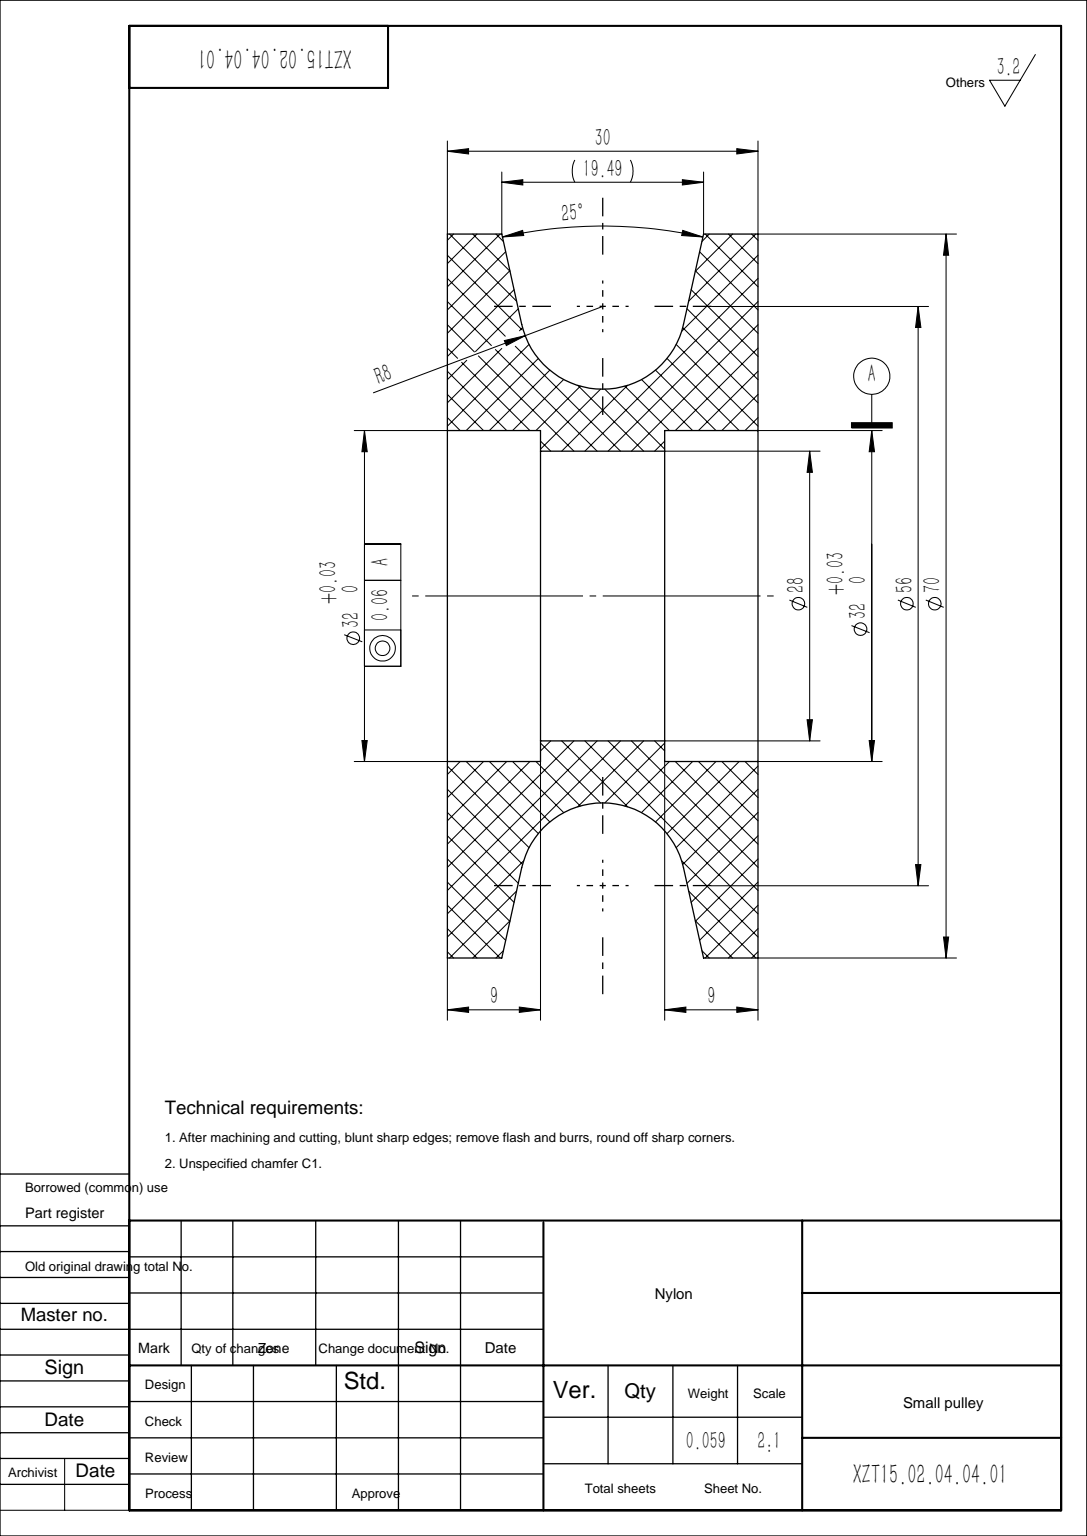
SolidWorks part; units mm, degrees
material "PA Type 6 Nylon"
ref_plane "Front Plane" through (0, 0, 0) normal (0, 0, 1) x (1, 0, 0)
ref_plane "Top Plane" through (0, 0, 0) normal (0, 1, 0) x (1, 0, 0)
ref_plane "Right Plane" through (0, 0, 0) normal (1, 0, 0) x (0, 0, -1)
sketch "Sketch1" plane through (0, 0, 0) normal (0, 0, 1) x (1, 0, 0)
  line L0 (-6, 14) -> (6, 14)
  line L1 (6, 14) -> (6, 16)
  line L2 (6, 16) -> (15, 16)
  line L3 (15, 16) -> (15, 35)
  line L4 (15, 35) -> (9.7461, 35)
  line L5 (9.7461, 35) -> (7.8104, 26.2685)
  line L6 (0, 14) -> (0, 20) construction
  line L7 (-9.7461, 35) -> (-7.8104, 26.2685)
  line L8 (-15, 35) -> (-9.7461, 35)
  line L9 (-15, 16) -> (-15, 35)
  line L10 (-6, 16) -> (-15, 16)
  line L11 (-6, 14) -> (-6, 16)
  line L12 (0, 0) -> (25.2987, 0) construction
  arc A0 (7.8104, 26.2685) -> (0, 20) centre (0, 28) cw
  arc A1 (-7.8104, 26.2685) -> (0, 20) centre (0, 28) ccw
  dimension "D1" = 70
  dimension "D6" = 8
  dimension "D2" = 28
  dimension "D3" = 32
  dimension "D4" = 30
  dimension "D5" = 25
  dimension "D7" = 9
  dimension "D8" = 56
revolve "Revolve1" add sketch "Sketch1" angle 360 about L12
